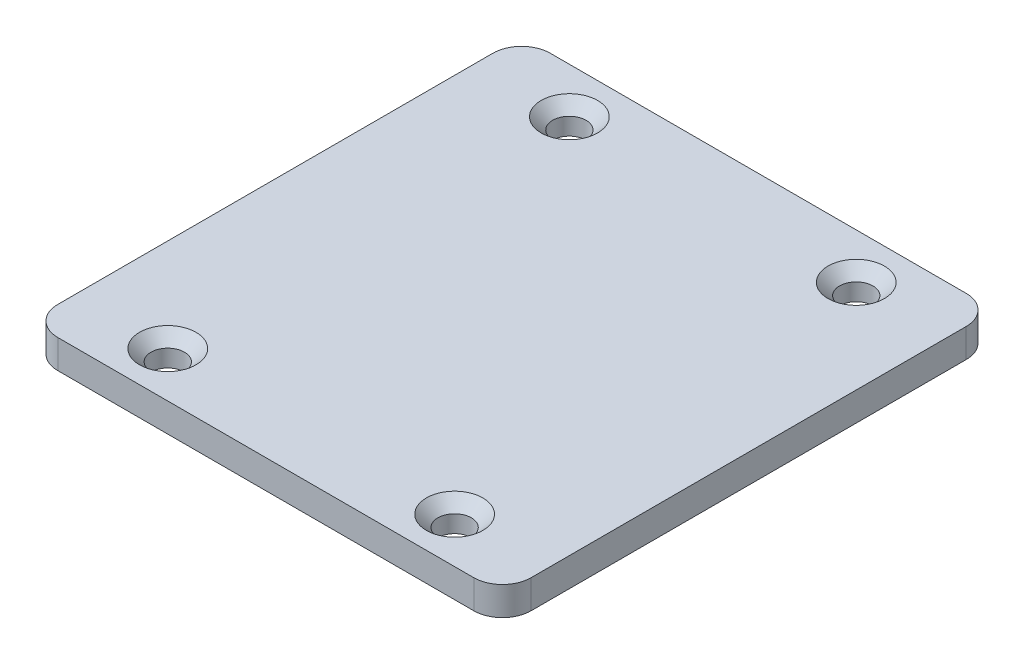
from build123d import *

# Parameters (mm, degrees)
SKETCH1_W           = 49.5
SKETCH1_H           = 51.5
SKETCH1_R           = 1.75
BOSS_EXTRUDE1_DEPTH = 3
CHAMFER1_SIZE       = 1.2
FILLET1_R           = 3


with BuildPart() as part:
    # Sketch1 → Boss-Extrude1 (new body)
    with BuildSketch(Plane(origin=(0, 0, 0), x_dir=(1, 0, 0), z_dir=(0, 1, 0))):
        Rectangle(SKETCH1_W, SKETCH1_H)
        with Locations(Location((-15, 21, 0), (0, 0, 270))):
            Circle(SKETCH1_R, mode=Mode.SUBTRACT)
        with Locations(Location((15, 21, 0), (0, 0, 270))):
            Circle(SKETCH1_R, mode=Mode.SUBTRACT)
        with Locations(Location((-15, -21, 0), (0, 0, 270))):
            Circle(SKETCH1_R, mode=Mode.SUBTRACT)
        with Locations(Location((15, -21, 0), (0, 0, 270))):
            Circle(SKETCH1_R, mode=Mode.SUBTRACT)
    extrude(amount=BOSS_EXTRUDE1_DEPTH)

    # Chamfer1
    chamfer1_edges = [part.edges().sort_by_distance(p)[0] for p in [
        (-15, 3, -22.75),
        (15, 3, -22.75),
        (-15, 3, 19.25),
        (15, 3, 19.25),
    ]]
    chamfer(chamfer1_edges, length=CHAMFER1_SIZE)

    # Fillet1
    fillet1_edges = [part.edges().sort_by_distance(p)[0] for p in [
        (24.75, 1.5, 25.75),
        (-24.75, 1.5, 25.75),
        (-24.75, 1.5, -25.75),
        (24.75, 1.5, -25.75),
    ]]
    fillet(fillet1_edges, radius=FILLET1_R)


solid = part.part
